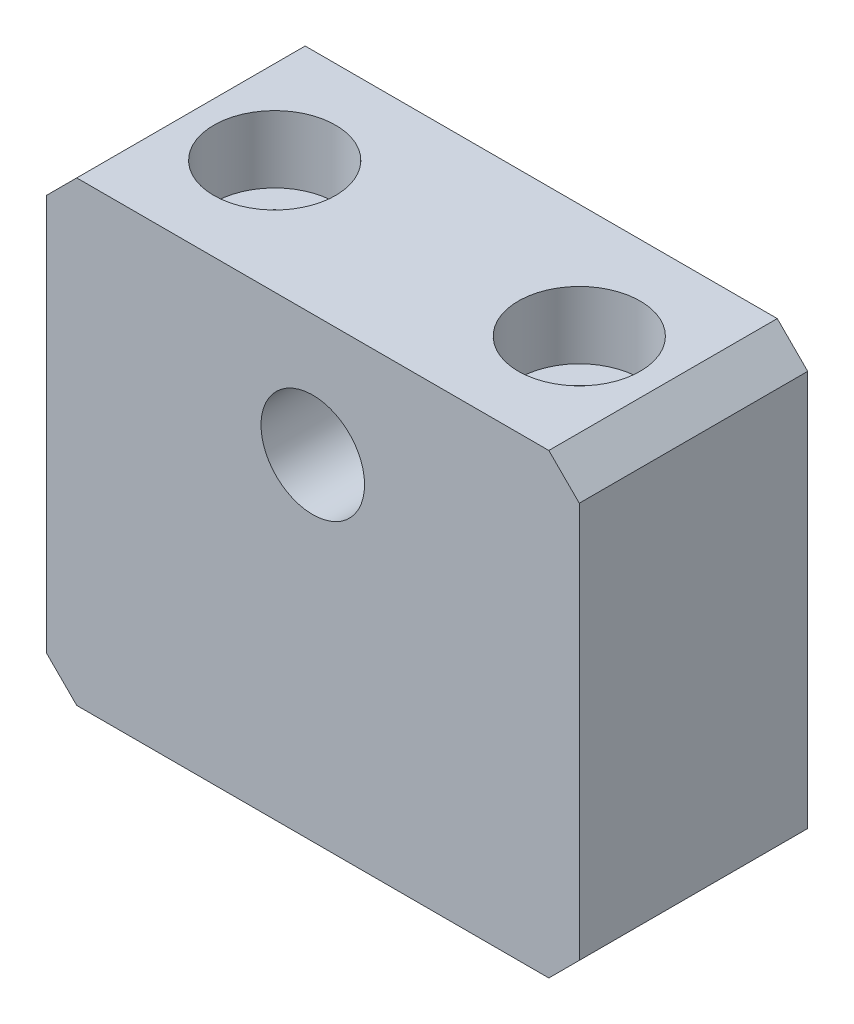
from build123d import *

# Parameters (mm, degrees)
SKETCH1_W                                           = 35
SKETCH1_H                                           = 30
BOSS_EXTRUDE1_DEPTH                                 = 15
CBORE_FOR_M4_HEX_SOCKET_HEAD_CAP_SCREW1_D           = 4.5
CBORE_FOR_M4_HEX_SOCKET_HEAD_CAP_SCREW1_CBORE_D     = 8
CBORE_FOR_M4_HEX_SOCKET_HEAD_CAP_SCREW1_CBORE_DEPTH = 4.4
M8_TAPPED_HOLE1_D                                   = 6.8
M8_TAPPED_HOLE1_DEPTH                               = 22.25
M8_TAPPED_HOLE1_TIP                                 = 2.042926105
CHAMFER1_SIZE                                       = 2


with BuildPart() as part:
    # Sketch1 → Boss-Extrude1 (new body)
    with BuildSketch(Plane.XY):
        Rectangle(SKETCH1_W, SKETCH1_H)
    extrude(amount=BOSS_EXTRUDE1_DEPTH)

    # CBORE for M4 Hex Socket Head Cap Screw1 (through all)
    with Locations(Plane(origin=(0, 15, 0), x_dir=(1, 0, 0), z_dir=(0, 1, 0))):
        with Locations((-10, -7.5), (10, -7.5)):
            CounterBoreHole(CBORE_FOR_M4_HEX_SOCKET_HEAD_CAP_SCREW1_D / 2, CBORE_FOR_M4_HEX_SOCKET_HEAD_CAP_SCREW1_CBORE_D / 2, CBORE_FOR_M4_HEX_SOCKET_HEAD_CAP_SCREW1_CBORE_DEPTH)

    # M8 Tapped Hole1
    with Locations(Plane.XY.offset(15)):
        with Locations((0, 7)):
            Hole(M8_TAPPED_HOLE1_D / 2, depth=M8_TAPPED_HOLE1_DEPTH)
            with Locations((0, 0, -(M8_TAPPED_HOLE1_DEPTH + M8_TAPPED_HOLE1_TIP / 2))):  # 118° drill point
                Cone(0, M8_TAPPED_HOLE1_D / 2, M8_TAPPED_HOLE1_TIP, mode=Mode.SUBTRACT)

    # Chamfer1
    chamfer1_edges = [part.edges().sort_by_distance(p)[0] for p in [
        (17.5, -15, 7.5),
        (-17.5, -15, 7.5),
        (-17.5, 15, 7.5),
        (17.5, 15, 7.5),
    ]]
    chamfer(chamfer1_edges, length=CHAMFER1_SIZE)


solid = part.part
